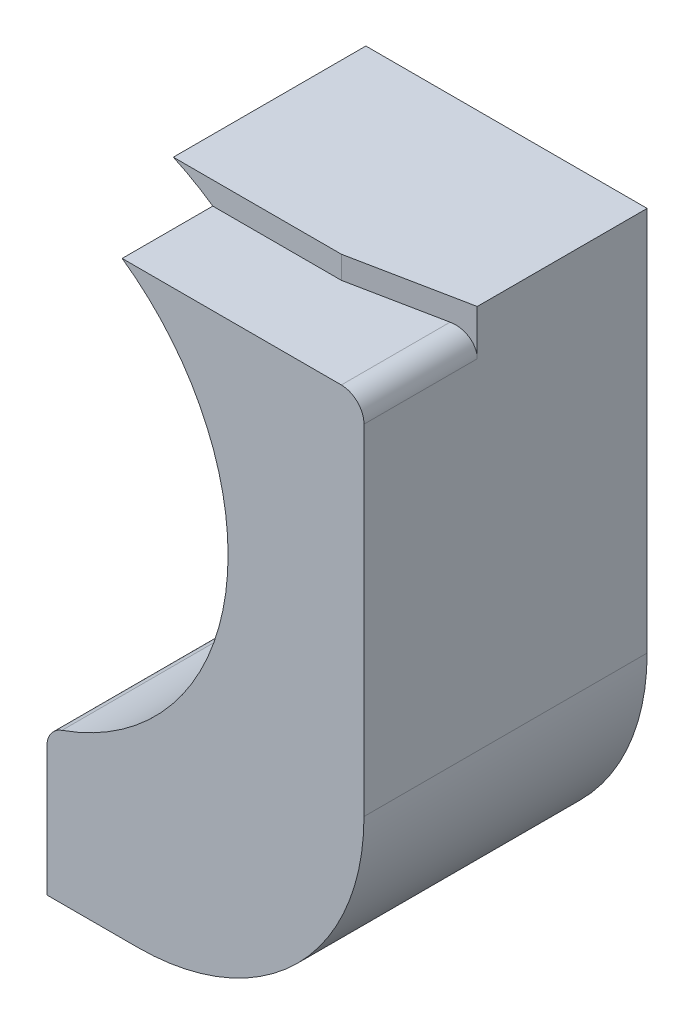
from build123d import *

# Parameters (mm, degrees)
EXTRUDE_1_DEPTH        = 12.5
CUT_EXTRUDE_1_DEPTH    = 1
FILLET_1_R             = 10
FILLET_2_R             = 1
HOLE_WIZARD_M2_1_D     = 1.6
HOLE_WIZARD_M2_1_DEPTH = 5.2
HOLE_WIZARD_M2_1_TIP   = 0.480688495
FILLET_4_R             = 1


with BuildPart() as part:
    # 草图1 → 凸台-拉伸1 (new body)
    with BuildSketch(Plane.XY):
        with BuildLine():
            Line((-7, -7.083005244), (-7, -13.5))
            Line((-7, -13.5), (7, -13.5))
            Line((7, -13.5), (7, 13.5))
            Line((7, 13.5), (-5.417424305, 13.5))
            ThreePointArc((-5.417424305, 13.5), (0.967629177, 2.656726476), (-7, -7.083005244))
        make_face()
    extrude(amount=EXTRUDE_1_DEPTH)

    # 草图2 → 切除-拉伸1 (cut)
    with BuildSketch(Plane(origin=(0, 13.5, 0), x_dir=(1, 0, 0), z_dir=(0, 1, 0))):
        Polygon((-5.417424305, -12.5), (-5.417424305, -8.5), (2, -8.5), (7, -7.5), (7, -12.5), align=None)
    extrude(amount=-CUT_EXTRUDE_1_DEPTH, mode=Mode.SUBTRACT)

    # 圆角1
    fillet_1_edges = [part.edges().sort_by_distance(p)[0] for p in [
        (7, -13.5, 6.25),
    ]]
    fillet(fillet_1_edges, radius=FILLET_1_R)

    # 圆角2
    fillet_2_edges = [part.edges().sort_by_distance(p)[0] for p in [
        (7, 12.5, 10),
    ]]
    fillet(fillet_2_edges, radius=FILLET_2_R)

    # M2 螺纹孔1
    with Locations(Plane(origin=(0, 0, 0), x_dir=(-1, 0, 0), z_dir=(0, 0, -1))):
        with Locations((-4, 2.5), (-4, 10.5)):
            Hole(HOLE_WIZARD_M2_1_D / 2, depth=HOLE_WIZARD_M2_1_DEPTH)
            with Locations((0, 0, -(HOLE_WIZARD_M2_1_DEPTH + HOLE_WIZARD_M2_1_TIP / 2))):  # 118° drill point
                Cone(0, HOLE_WIZARD_M2_1_D / 2, HOLE_WIZARD_M2_1_TIP, mode=Mode.SUBTRACT)

    # 圆角4
    fillet_4_edges = [part.edges().sort_by_distance(p)[0] for p in [
        (-7, -7.083005244, 6.25),
    ]]
    fillet(fillet_4_edges, radius=FILLET_4_R)


solid = part.part
